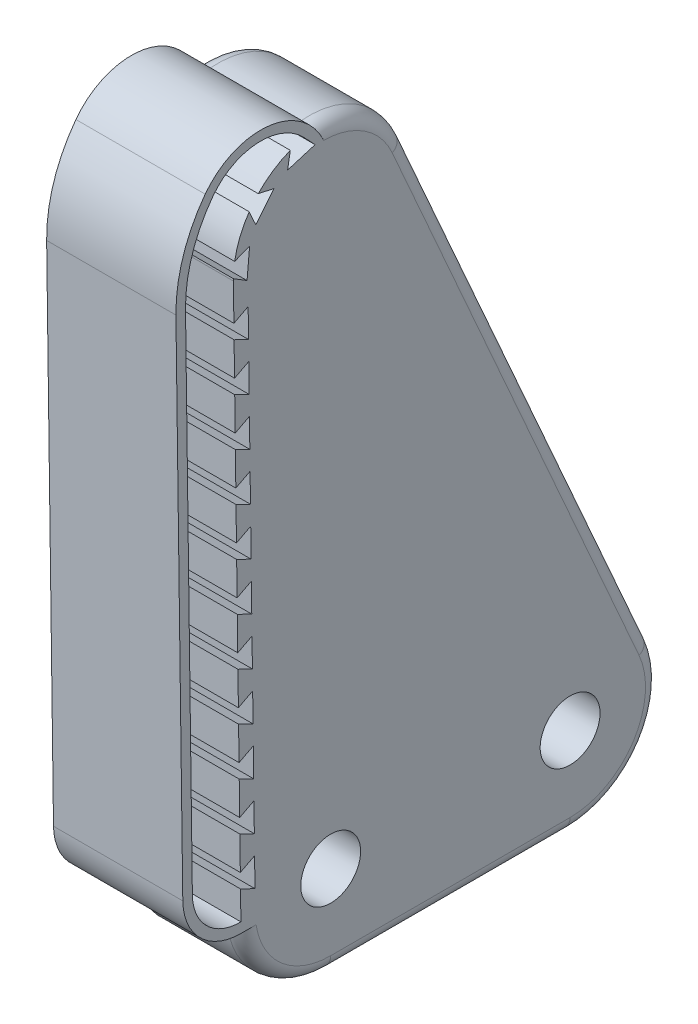
SolidWorks part; units mm, degrees
material "ABS"
ref_plane "Front" through (0, 0, 0) normal (0, 0, 1) x (1, 0, 0)
ref_plane "Top" through (0, 0, 0) normal (0, 1, 0) x (1, 0, 0)
ref_plane "Right" through (0, 0, 0) normal (1, 0, 0) x (0, 0, -1)
sketch "Sketch1" plane through (0, 0, 0) normal (1, 0, 0) x (0, 0, -1)
  line L0 (0, -4.7625) -> (12.7, -4.7625)
  line L1 (17.0561, 1.9251) -> (3.9577, 31.5642)
  line L2 (-5.1604, 29.5751) -> (-4.7621, -0.064)
  arc A0 (-4.7621, -0.064) -> (0, -4.7625) centre (0, 0) ccw
  arc A1 (12.7, -4.7625) -> (17.0561, 1.9251) centre (12.7, 0) ccw
  arc A2 (3.9577, 31.5642) -> (-5.1604, 29.5751) centre (-0.3983, 29.6391) ccw
  dimension "D1" = 4.7625
  dimension "D2" = 12.7
  dimension "D3" = 29.6418
  dimension "D4" = 90.77
extrude "Boss-Extrude1" add sketch "Sketch1" along normal blind 6.35
sketch "Sketch2" plane through (6.35, 0, 0) normal (1, 0, 0) x (0, 0, -1)
  circle A1 centre (0, 0) radius 1.5875
  circle A2 centre (12.7, 0) radius 1.5875
  dimension "D1" = 3.175
extrude "Cut-Extrude1" cut sketch "Sketch2" against normal blind 38.1
sketch "Sketch3" plane through (6.35, 0, 0) normal (1, 0, 0) x (0, 0, -1)
  line L0 (-4.7826, 1.4599) -> (-4.7928, 2.2218)
  line L1 (-5.1604, 29.5751) -> (-4.7621, -0.064) construction
  line L2 (-4.7928, 2.2218) -> (-4.036, 2.613)
  line L3 (-4.036, 2.613) -> (-4.0155, 1.0891)
  line L4 (-4.0155, 1.0891) -> (-4.7826, 1.4599)
  dimension "D1" = 0.762
  dimension "D2" = 1.524
  dimension "D3" = 0.762
  dimension "D4" = 1.524
extrude "Cut-Extrude2" cut sketch "Sketch3" against normal blind 6.35
pattern_linear "LPattern1" count 11 spacing 2.54 along (0, 0.9999, 0.0134) of "Cut-Extrude2"
sketch "Sketch5" plane through (6.35, 0, 0) normal (1, 0, 0) x (0, 0, -1)
  line L0 (-2.1425, 34.0708) -> (-2.2856, 33.2309)
  line L1 (-2.2856, 33.2309) -> (-0.8274, 33.6738)
  line L2 (-0.8274, 33.6738) -> (-1.4134, 34.2922)
  line L3 (-2.1425, 34.0708) -> (-1.4134, 34.2922) construction
  arc A0 (3.9577, 31.5642) -> (-5.1604, 29.5751) centre (-0.3983, 29.6391) ccw construction
  arc A1 (-2.1425, 34.0708) -> (-1.4134, 34.2922) centre (-0.3983, 29.6391) cw
  dimension "D1" = 0.762
  dimension "D2" = 1.524
  dimension "D3" = 0.762
extrude "Cut-Extrude3" cut sketch "Sketch5" against normal blind 6.35
pattern_circular "CirPattern1" count 3 every 34 about axis through (0, 29.6391, 0.3983) along (1, 0, 0) of "Cut-Extrude3"
sketch "Sketch6" plane through (0, 0, 0) normal (1, 0, 0) x (0, 0, -1)
  line L0 (0, 0) -> (-4.7621, -0.064) construction
  line L1 (-7.336, 2.4416) -> (-7.7002, 29.541)
  line L2 (-0.8274, 33.6738) -> (-1.4134, 34.2922) construction
  line L3 (-8.2081, 29.5342) -> (-7.844, 2.4416)
  line L4 (-4.7621, -0.5992) -> (-4.7247, -0.5992)
  line L6 (-4.7826, 1.4599) -> (-4.7621, -0.064) construction
  arc A0 (-4.7621, -0.064) -> (-7.336, 2.4416) centre (-4.7962, 2.4758) cw
  arc A1 (-7.7002, 29.541) -> (-6.2491, 34.009) centre (-0.3983, 29.6391) cw
  arc A2 (3.9577, 31.5642) -> (-1.4134, 34.2922) centre (-0.3983, 29.6391) ccw construction
  arc A3 (-1.4134, 34.2922) -> (-6.2491, 34.009) centre (-3.7119, 32.114) ccw
  arc A4 (-1.4134, 34.2922) -> (-0.8213, 34.3828) centre (-0.3983, 29.6391) cw
  arc A5 (-0.8213, 34.3828) -> (-6.6561, 34.313) centre (-3.7119, 32.114) ccw
  arc A6 (-6.6561, 34.313) -> (-8.2081, 29.5342) centre (-0.3983, 29.6391) ccw
  arc A7 (-7.844, 2.4416) -> (-4.7621, -0.5992) centre (-4.7621, 2.4831) ccw
  arc A9 (-4.7621, -0.064) -> (0, -4.7625) centre (0, 0) ccw construction
  arc A10 (-4.7621, -0.064) -> (-4.7247, -0.5992) centre (0, 0) ccw
  dimension "D1" = 2.54
  dimension "D2" = 0.508
extrude "Boss-Extrude2" add sketch "Sketch6" along normal blind 6.35
sketch "Sketch7" plane through (0, 0, 0) normal (-1, 0, 0) x (0, 0, 1)
  line L0 (3.8905, 29.5922) -> (3.4848, -0.5992)
  line L1 (4.0155, 1.0891) -> (4.036, 2.613) construction
  line L2 (4.7621, -0.5992) -> (3.4848, -0.5992)
  line L3 (7.844, 2.4416) -> (8.2081, 29.5342)
  line L4 (0.8213, 34.3828) -> (-0.2014, 33.0797)
  arc A0 (4.7621, -0.5992) -> (7.844, 2.4416) centre (4.7621, 2.4831) ccw
  arc A1 (8.2081, 29.5342) -> (6.6561, 34.313) centre (0.3983, 29.6391) ccw
  arc A2 (6.6561, 34.313) -> (0.8213, 34.3828) centre (3.7119, 32.114) ccw
  arc A3 (-0.2014, 33.0797) -> (3.8905, 29.5922) centre (0.3983, 29.6391) cw
  dimension "D1" = 0.508
extrude "Boss-Extrude3" add sketch "Sketch7" along normal blind 0.508
fillet "Fillet3" radius 0.762 10 edges at (6.35, -3.5732, 3.1486) (6.35, -4.7625, -6.35) (6.35, 33.7413, -2.0211) (6.35, 16.7446, -10.5069) (0, -3.5732, 3.1486) (0, -4.7625, -6.35) (0, 33.7413, -2.0211) (0, 16.7446, -10.5069) (6.35, -2.5993, -16.6906) (0, -2.5993, -16.6906)
scale "Scale ratio 1" scale about origin uniform scaling yes scale factor 1.3
